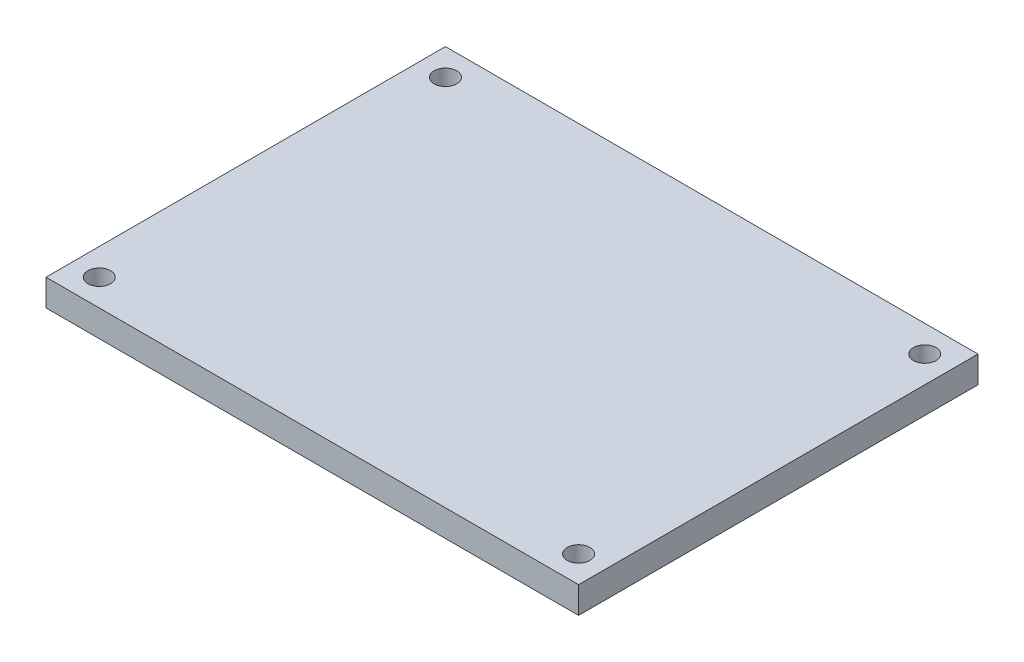
SolidWorks part; units mm, degrees
ref_plane "前视基准面" through (0, 0, 0) normal (0, 0, 1) x (1, 0, 0)
ref_plane "上视基准面" through (0, 0, 0) normal (0, 1, 0) x (1, 0, 0)
ref_plane "右视基准面" through (0, 0, 0) normal (1, 0, 0) x (0, 0, -1)
sketch "草图1" plane through (0, 0, 0) normal (0, 1, 0) x (1, 0, 0)
  line L1 (-100, 75) -> (100, 75)
  line L2 (-100, 75) -> (-100, -75)
  line L3 (-100, -75) -> (100, -75)
  line L4 (100, 75) -> (100, -75)
  line L5 (-100, 75) -> (100, -75) construction
  line L6 (-100, -75) -> (100, 75) construction
  point P0 (0, 0)
  dimension "D1" = 200
  dimension "D2" = 150
extrude "凸台-拉伸1" add sketch "草图1" along normal blind 10
hole_wizard "M10 螺纹孔1" positions "草图2" profile "草图3" tap size "M10" standard "GB" end condition through all
sketch "草图2" plane through (0, 0, 0) normal (0, -1, 0) x (-1, 0, 0)
  line L0 (0, 0) -> (0, -72.8439) construction
  line L3 (0, 0) -> (-75.8277, 0) construction
  line L6 (100, 75) -> (100, -75) construction
  line L7 (100, -75) -> (-100, -75) construction
  point P0 (90, -65)
  point P2 (90, 65)
  point P4 (-90, 65)
  point P6 (-90, -65)
  dimension "D1" = 10
  dimension "D2" = 10
sketch "草图3" plane through (-90, 0, 65) normal (1, 0, 0) x (0, 0, -1)
  line L0 (0, 0) -> (0, 10)
  line L1 (0, 10) -> (4.25, 10)
  line L2 (4.25, 10) -> (4.25, 0)
  line L5 (4.25, 0) -> (0, 0)
  line L11 (0, -6.35) -> (0, 107.95) construction
  dimension "通孔螺纹孔钻头直径" = 8.5
  dimension "通孔螺纹孔钻头深度" = 10
cosmetic thread "孔螺蚊线1" parameters "D2"=10
cosmetic thread "孔螺蚊线2" parameters "D2"=10
cosmetic thread "孔螺蚊线3" parameters "D2"=10
cosmetic thread "孔螺蚊线4" parameters "D2"=10
